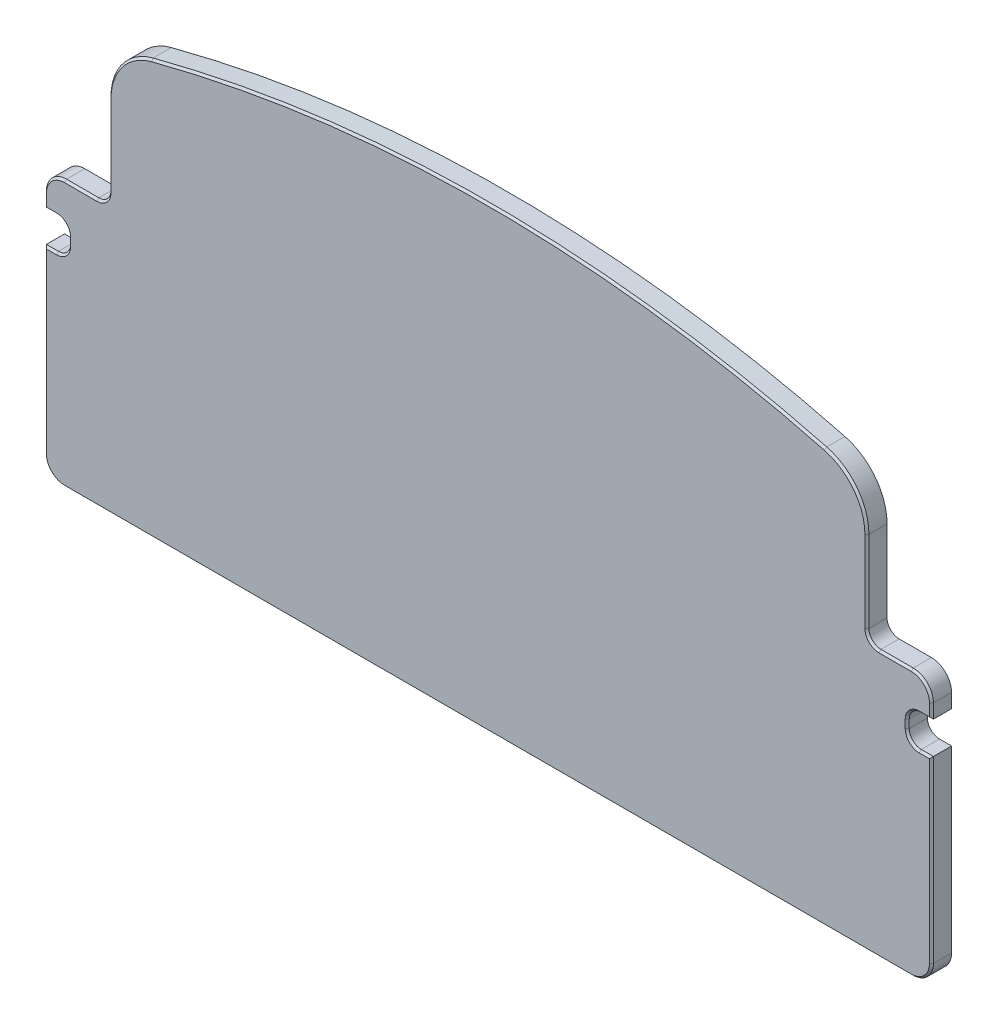
SolidWorks part; units mm, degrees
material "6061 合金"
ref_plane "前视基准面" through (0, 0, 0) normal (0, 0, 1) x (1, 0, 0)
ref_plane "上视基准面" through (0, 0, 0) normal (0, 1, 0) x (1, 0, 0)
ref_plane "右视基准面" through (0, 0, 0) normal (1, 0, 0) x (0, 0, -1)
sketch "草图1" plane through (0, 0, 0) normal (0, 0, 1) x (1, 0, 0)
  line L1 (-110, 121) -> (110, 121)
  line L2 (-110, 121) -> (-110, 0)
  line L3 (-110, 0) -> (110, 0)
  line L4 (110, 121) -> (110, 0)
  dimension "D1" = 220
  dimension "D2" = 121
extrude "凸台-拉伸1" add sketch "草图1" along normal mid plane 5
sketch "草图4" plane through (0, 0, 2.5) normal (0, 0, 1) x (1, 0, 0)
  line L4 (-94, 66) -> (-110, 66)
  line L5 (-110, 125.2) -> (110, 125.2)
  line L6 (110, 125.2) -> (110, 66)
  line L7 (-94, 66) -> (-94, 89.2057)
  line L8 (94, 66) -> (94, 89.2057)
  line L11 (0, 74) -> (67.5, 74) construction
  line L12 (0, 0) -> (0, 75) construction
  line L13 (110, 66) -> (94, 66)
  line L14 (-110, 66) -> (-110, 125.2)
  line L15 (-110, 121) -> (-110, 0) construction
  line L16 (110, 0) -> (110, 121) construction
  line L17 (-110, 0) -> (110, 0) construction
  arc A1 (-83.5443, 102.7497) -> (-94, 89.2057) centre (-80, 89.2057) ccw
  arc A2 (83.5443, 102.7497) -> (94, 89.2057) centre (80, 89.2057) cw
  arc A3 (83.5443, 102.7497) -> (-83.5443, 102.7497) centre (0, -216.5) ccw
  dimension "D3" = 14
  dimension "D5" = 330
  dimension "D1" = 59.2
  dimension "D2" = 188
  dimension "D8" = 216.5
  dimension "D10" = 66
extrude "切除-拉伸1" cut sketch "草图4" against normal through all
sketch "草图5" plane through (0, 0, 2.5) normal (0, 0, 1) x (1, 0, 0)
  line L0 (-110, 66) -> (-110, 0) construction
  line L1 (-110, 57.5) -> (-104, 57.5)
  line L2 (-110, 57.5) -> (-110, 49.5)
  line L3 (-110, 49.5) -> (-104, 49.5)
  line L4 (-104, 57.5) -> (-104, 49.5)
  line L5 (110, 0) -> (110, 66) construction
  line L6 (110, 57.5) -> (104, 57.5)
  line L7 (110, 57.5) -> (110, 49.5)
  line L8 (110, 49.5) -> (104, 49.5)
  line L9 (104, 57.5) -> (104, 49.5)
  line L10 (0, 0) -> (0, 75) construction
  line L12 (104, 53.5) -> (-104, 53.5) construction
  line L13 (-110, 0) -> (110, 0) construction
  dimension "D1" = 53.5
  dimension "D2" = 8
  dimension "D3" = 208
extrude "切除-拉伸2" cut sketch "草图5" against normal through all
fillet "圆角1" radius 5 4 edges at (-110, 0, 0) (110, 0, 0) (-110, 66, 0) (110, 66, 0)
fillet "圆角2" radius 3 6 edges at (-104, 49.5, 0) (-104, 57.5, 0) (104, 49.5, 0) (104, 57.5, 0) (-94, 66, 0) (94, 66, 0)
chamfer "倒角1" distance 0.5 angle 45 28 edges at (110, 27.25, 2.5) (108.5355, 1.4645, 2.5) (0, 0, 2.5) (-108.5355, 1.4645, 2.5) (108.5, 57.5, 2.5) (110, 59.25, 2.5) (108.5355, 64.5355, 2.5) (101, 66, 2.5) (94, 79.1029, 2.5) (91.082, 97.7608, 2.5) (0, 113.5, 2.5) (-91.082, 97.7608, 2.5) (-94, 79.1029, 2.5) (-101, 66, 2.5) (-108.5355, 64.5355, 2.5) (-110, 59.25, 2.5) (-108.5, 57.5, 2.5) (-104, 53.5, 2.5) (-108.5, 49.5, 2.5) (-110, 27.25, 2.5) (108.5, 49.5, 2.5) (104, 53.5, 2.5) (104.8787, 56.6213, 2.5) (-104.8787, 56.6213, 2.5) (104.8787, 50.3787, 2.5) (-104.8787, 50.3787, 2.5) (94.8787, 66.8787, 2.5) (-94.8787, 66.8787, 2.5)
